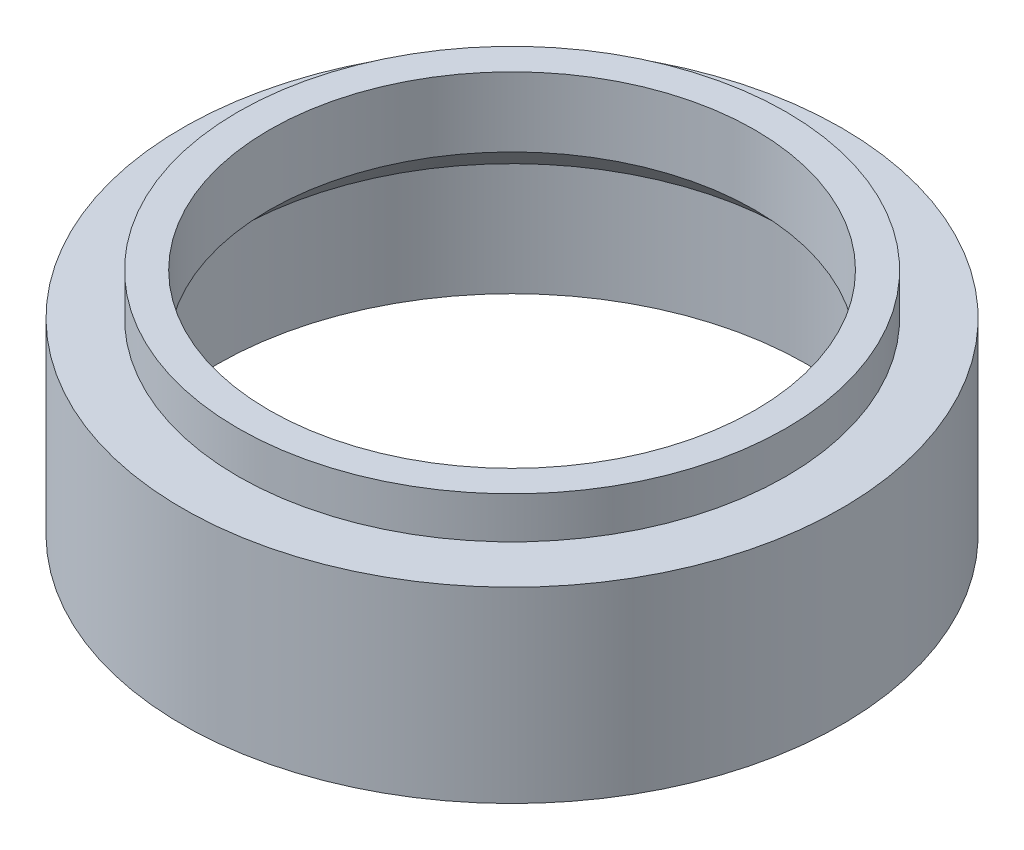
from build123d import *

# Parameters (mm, degrees)
CHAMFER_1_SIZE = 5


with BuildPart() as part:
    # 草图2 → 旋转1 (revolve)
    with BuildSketch(Plane.XY, mode=Mode.PRIVATE) as revolve_1_sk:
        Polygon((-35, 33), (-39.5, 33), (-39.5, 27), (-47.5, 27), (-47.5, 0), (-42.5, 0), (-42.5, 18), (-35, 18), align=None)
    revolve(revolve_1_sk.sketch.rotate(Axis((0, 0, 0), (0, 1, 0)), 270), axis=Axis((0, 0, 0), (0, 1, 0)))

    # 倒角1
    chamfer_1_edges = [part.edges().sort_by_distance(p)[0] for p in [
        (0, 18, 35),
    ]]
    chamfer(chamfer_1_edges, length=CHAMFER_1_SIZE)


solid = part.part
